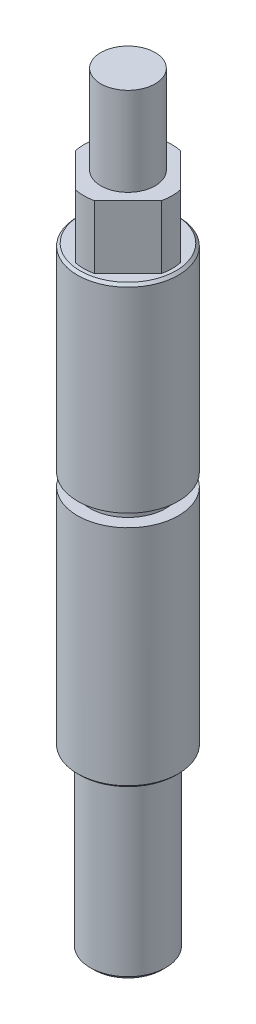
SolidWorks part; units mm, degrees
ref_plane "Front Plane" through (0, 0, 0) normal (0, 0, 1) x (1, 0, 0)
ref_plane "Top Plane" through (0, 0, 0) normal (0, 1, 0) x (1, 0, 0)
ref_plane "Right Plane" through (0, 0, 0) normal (1, 0, 0) x (0, 0, -1)
ref_plane "Plane4" through (0, 0, 0) normal (0, 0, -1) x (-1, 0, 0)
sketch "Sketch1" plane through (0, 0, 0) normal (0, 0, -1) x (-1, 0, 0)
  line L0 (-4, -29.4953) -> (0, -29.4953)
  line L1 (0, -29.4953) -> (0, 5.1)
  line L2 (0, 5.1) -> (-4, 5.1)
  line L3 (-4, 5.1) -> (-4, -10.6)
  line L4 (-4, -10.6) -> (-3, -10.6)
  line L5 (-3, -10.6) -> (-3, -11.6)
  line L6 (-3, -11.6) -> (-4, -11.6)
  line L7 (-4, -11.6) -> (-4, -29.4953)
  line L8 (0, -29.4953) -> (0, 5.1) construction
revolve "Revolve1" add sketch "Sketch1" angle 360 about L8
sketch "Sketch2" plane through (0, -29.4953, 0) normal (0, -1, 0) x (1, 0, 0)
  circle A0 centre (0, 0) radius 3
extrude "Boss-Extrude1" add sketch "Sketch2" along normal blind 13.9047
sketch "Sketch3" plane through (0, 5.1, 0) normal (0, 1, 0) x (-1, 0, 0)
  line L0 (3.4178, -0.7541) -> (0.7541, -3.4178)
  line L1 (-0.7541, -3.4178) -> (-3.4178, -0.7541)
  line L2 (-3.4178, 0.7541) -> (-0.7541, 3.4178)
  line L3 (0.7541, 3.4178) -> (3.4178, 0.7541)
  arc A0 (0.7541, -3.4178) -> (-0.7541, -3.4178) centre (0, 0) cw
  arc A1 (-3.4178, -0.7541) -> (-3.4178, 0.7541) centre (0, 0) cw
  arc A2 (-0.7541, 3.4178) -> (0.7541, 3.4178) centre (0, 0) cw
  arc A3 (3.4178, 0.7541) -> (3.4178, -0.7541) centre (0, 0) cw
extrude "Boss-Extrude2" add sketch "Sketch3" along normal blind 5
sketch "Sketch4" plane through (0, 10.1, 0) normal (0, 1, 0) x (-1, 0, 0)
  circle A0 centre (0, 0) radius 2.15
extrude "Boss-Extrude3" add sketch "Sketch4" along normal blind 7
chamfer "Chamfer1" distance 0.2 angle 45 2 edges at (0, -29.4953, 4) (0, 5.1, 4)
chamfer "Chamfer2" distance 0.3 angle 45 1 edges at (0, -43.4, -3)
